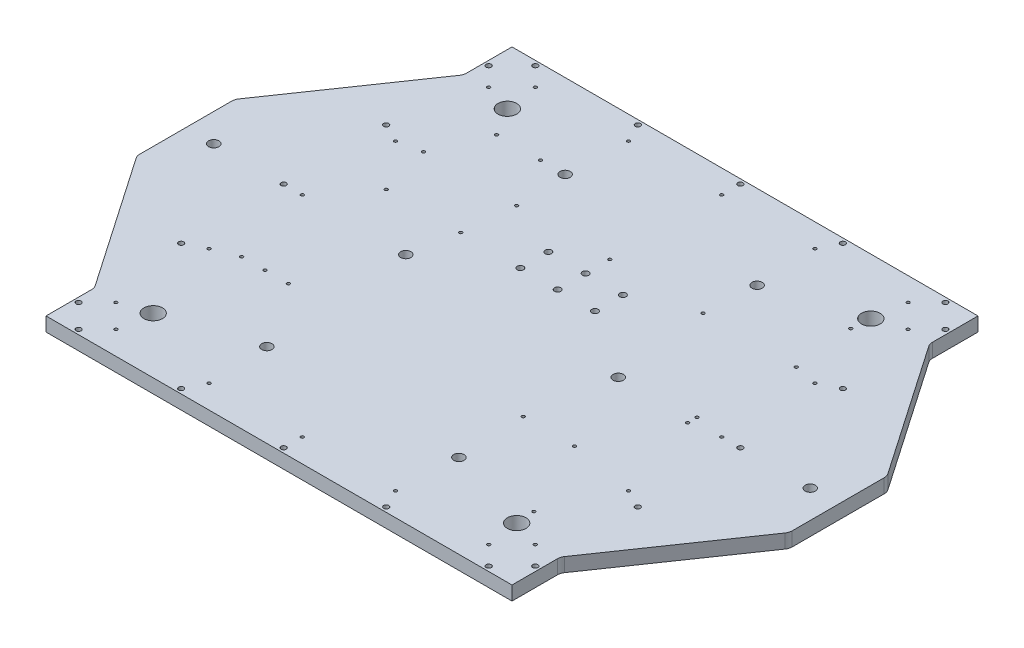
from build123d import *

# Parameters (mm, degrees)
SKETCH_1_W                   = 700
SKETCH_1_H                   = 500
EXTRUDE_1_DEPTH              = 15
CUT_EXTRUDE_1_DEPTH          = 431.37774106
HOLE_WIZARD_M5_2_D           = 5.5
HOLE_WIZARD_M5_2_CBORE_D     = 9.9
HOLE_WIZARD_M5_2_CBORE_DEPTH = 5.4
HOLE_WIZARD_M10_1_D          = 11
SKETCH_9_R                   = 10
CUT_EXTRUDE_2_DEPTH          = 431.37774106
HOLE_WIZARD_M8_2_D           = 6.8
HOLE_WIZARD_M4_1_D           = 3.3
HOLE_WIZARD_M4_2_D           = 3.3
FILLET_1_R                   = 10


with BuildPart() as part:
    # 草图1 → 凸台-拉伸1 (new body)
    with BuildSketch(Plane(origin=(0, 0, 0), x_dir=(1, 0, 0), z_dir=(0, 1, 0))):
        Rectangle(SKETCH_1_W, SKETCH_1_H)
    extrude(amount=EXTRUDE_1_DEPTH)

    # 草图2 → 切除-拉伸1 (cut, through all)
    with BuildSketch(Plane(origin=(0, 15, 0), x_dir=(1, 0, 0), z_dir=(0, 1, 0))):
        Polygon((-250, 250), (-250, 198), (-350, 52.5), (-350, 250), align=None)
        Polygon((350, 250), (250, 250), (250, 198), (350, 52.5), align=None)
        Polygon((250, -250), (250, -198), (350, -52.5), (350, -250), align=None)
        Polygon((-350, -250), (-250, -250), (-250, -198), (-350, -52.5), align=None)
    extrude(amount=-CUT_EXTRUDE_1_DEPTH, mode=Mode.SUBTRACT)

    # M5 六角凹头螺钉的柱形沉头孔2 (through all)
    with Locations(Plane(origin=(0, 0, 0), x_dir=(-1, 0, 0), z_dir=(0, -1, 0))):
        with Locations((-220, 245), (-110, 245), (0, 245), (110, 245), (220, 245), (245, 220), (245, 110), (245, 0), (245, -110), (245, -220), (220, -245), (110, -245), (0, -245), (-110, -245), (-220, -245), (-245, -220), (-245, -110), (-245, 0), (-245, 110), (-245, 220)):
            CounterBoreHole(HOLE_WIZARD_M5_2_D / 2, HOLE_WIZARD_M5_2_CBORE_D / 2, HOLE_WIZARD_M5_2_CBORE_DEPTH)

    # M10 间隙孔1 (through all)
    with Locations(Plane(origin=(0, 0, 0), x_dir=(-1, 0, 0), z_dir=(0, -1, 0))):
        with Locations((-320, 0), (-114, 0), (114, 0), (320, 0), (-103, 160), (103, 160), (103, -160), (-103, -160)):
            Hole(HOLE_WIZARD_M10_1_D / 2)

    # 草图9 → 切除-拉伸2 (cut, through all)
    with BuildSketch(Plane.XZ):
        with Locations(Location((195, 190, 0), (0, 0, 270))):
            Circle(SKETCH_9_R)
        with Locations(Location((195, -190, 0), (0, 0, 270))):
            Circle(SKETCH_9_R)
        with Locations(Location((-195, -190, 0), (0, 0, 270))):
            Circle(SKETCH_9_R)
        with Locations(Location((-195, 190, 0), (0, 0, 270))):
            Circle(SKETCH_9_R)
    extrude(amount=-CUT_EXTRUDE_2_DEPTH, mode=Mode.SUBTRACT)

    # M8 螺纹孔2 (through all)
    with Locations(Plane(origin=(0, 15, 0), x_dir=(1, 0, 0), z_dir=(0, 1, 0))):
        with Locations((-40, 79), (0, 79), (40, 79), (40, 49), (0, 49), (-40, 49)):
            Hole(HOLE_WIZARD_M8_2_D / 2)

    # M4 螺纹孔1 (through all)
    with Locations(Plane(origin=(0, 15, 0), x_dir=(1, 0, 0), z_dir=(0, 1, 0))):
        with Locations((0, 225), (100, 225), (200, 225), (-200, 225), (-100, 225), (225, 0), (225, 100), (225, 200), (225, -200), (225, -100), (-225, -100), (-225, -200), (-225, 200), (-225, 100), (-225, 0), (-100, -225), (-200, -225), (200, -225), (100, -225), (0, -225), (0, 105), (100, 105), (200, 105), (-200, 105), (-100, 105)):
            Hole(HOLE_WIZARD_M4_1_D / 2)

    # M4 螺纹孔2 (through all)
    with Locations(Plane(origin=(0, 15, 0), x_dir=(1, 0, 0), z_dir=(0, 1, 0))):
        with Locations((-185, 50), (-105, 50), (-176.5, 160), (-129.5, 160), (193.5, 170), (193.5, 5), (193.5, -5), (193.5, -170), (99.5, -87.5), (154.5, -87.5), (-150, -90), (-200, -90), (-175, -90)):
            Hole(HOLE_WIZARD_M4_2_D / 2)

    # 圆角1
    fillet_1_edges = [part.edges().sort_by_distance(p)[0] for p in [
        (-350, 7.5, 52.5),
        (-250, 7.5, 198),
        (250, 7.5, 198),
        (350, 7.5, 52.5),
        (350, 7.5, -52.5),
        (250, 7.5, -198),
        (-250, 7.5, -198),
        (-350, 7.5, -52.5),
    ]]
    fillet(fillet_1_edges, radius=FILLET_1_R)


solid = part.part
